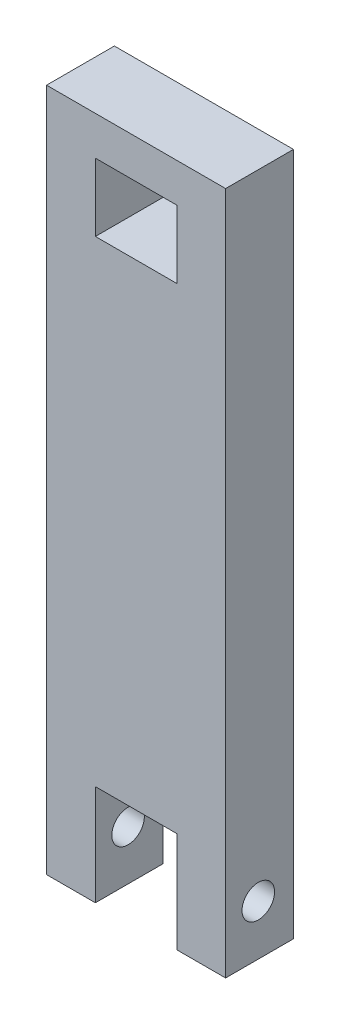
from build123d import *

# Parameters (mm, degrees)
EXTRUDE_1_DEPTH          = 12.5
HOLE_WIZARD_M14_1_D      = 12
HOLE_WIZARD_M14_1_DEPTH  = 18
SKETCH_7_W               = 66
SKETCH_7_H               = 25
EXTRUDE_2_DEPTH          = 12
CUT_EXTRUDE_5_DEPTH      = 156.608483059
CUT_EXTRUDE_5_DEPTH_BACK = 156.608483059
SKETCH_12_W              = 30
SKETCH_12_H              = 25


with BuildPart() as part:
    # 草图1 → 凸台-拉伸1 (new, symmetric)
    with BuildSketch(Plane.XY):
        Polygon((-33, -150), (-15, -150), (-15, -112.904160338), (0, -112.904160338), (15, -112.904160338), (15, -150), (33, -150), (33, 90), (15, 90), (-15, 90), (-33, 90), align=None)
    extrude(amount=EXTRUDE_1_DEPTH, both=True)

    # M14 螺纹孔1
    with Locations(Plane(origin=(33, -131.5, 0.451602972), x_dir=(0, 0, 1), z_dir=(1, 0, 0))):
        with Locations((0, 0)):
            hole_wizard_m14_1 = Hole(HOLE_WIZARD_M14_1_D / 2, depth=HOLE_WIZARD_M14_1_DEPTH)

    # 镜向1: M14 螺纹孔1 across plane
    add(hole_wizard_m14_1.mirror(Plane(origin=(0, 0, 0), x_dir=(0, 0, 1), z_dir=(1, 0, 0))), mode=Mode.SUBTRACT)

    # 草图7 → 凸台-拉伸2 (add)
    with BuildSketch(Plane(origin=(0, 90, 0), x_dir=(1, 0, 0), z_dir=(0, 1, 0))):
        Rectangle(SKETCH_7_W, SKETCH_7_H)
    extrude(amount=EXTRUDE_2_DEPTH)

    # 草图12 → 切除-拉伸5 (cut, two sides: drawn at the far end of the back side and taken through both)
    with BuildSketch(Plane(origin=(0, 0, -12.5), x_dir=(-1, 0, 0), z_dir=(0, 0, -1)).offset(-CUT_EXTRUDE_5_DEPTH_BACK)):
        with Locations((0, 75.204537633)):
            Rectangle(SKETCH_12_W, SKETCH_12_H)
    extrude(amount=CUT_EXTRUDE_5_DEPTH + CUT_EXTRUDE_5_DEPTH_BACK, mode=Mode.SUBTRACT)


solid = part.part
